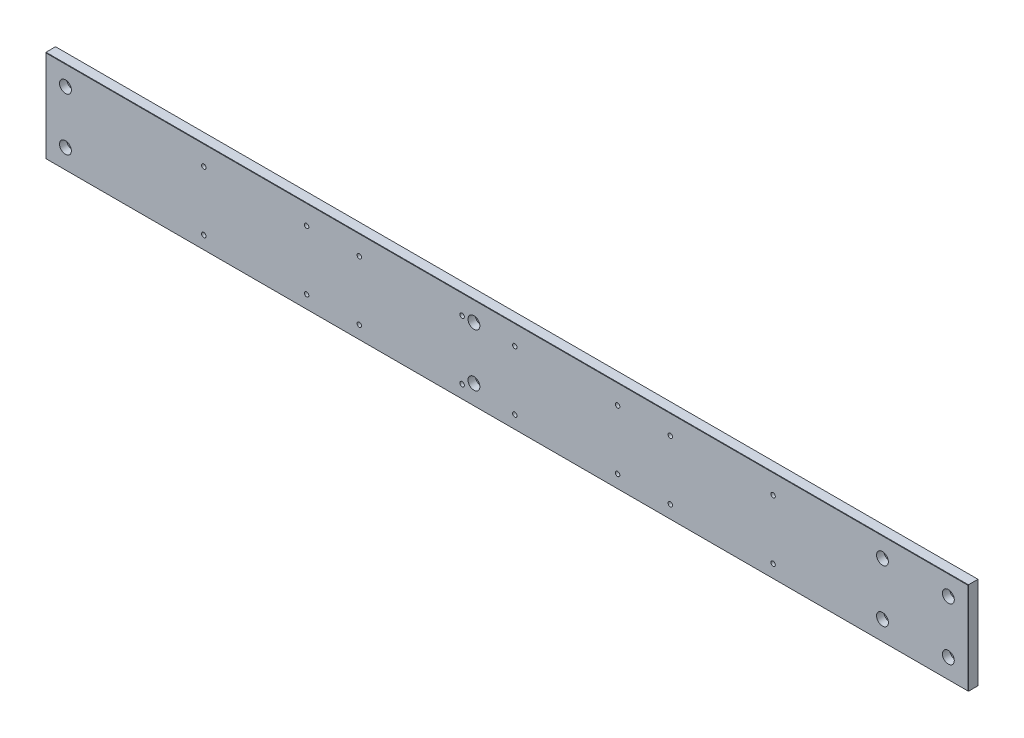
SolidWorks part; units mm, degrees
material "普通碳钢"
ref_plane "前视基准面" through (0, 0, 0) normal (0, 0, 1) x (1, 0, 0)
ref_plane "上视基准面" through (0, 0, 0) normal (0, 1, 0) x (1, 0, 0)
ref_plane "右视基准面" through (0, 0, 0) normal (1, 0, 0) x (0, 0, -1)
sketch "草图1" plane through (0, 0, 0) normal (0, 0, 1) x (1, 0, 0)
  line L1 (-700, 70) -> (700, 70)
  line L2 (-700, 70) -> (-700, -70)
  line L3 (-700, -70) -> (700, -70)
  line L4 (700, 70) -> (700, -70)
  line L5 (-700, 70) -> (700, -70) construction
  line L6 (-700, -70) -> (700, 70) construction
  point P0 (0, 0)
  dimension "D1" = 1400
  dimension "D2" = 140
extrude "凸台-拉伸1" add sketch "草图1" along normal mid plane 15
hole_wizard "打孔尺寸(%根据)内六角圆柱头螺钉的类型1" positions "3D草图1" profile "草图2" counterbore size "M10" standard "GB" end condition through all
sketch3d "3D草图1"
  line L0 (700, 70, 7.5) -> (-700, 70, 7.5) construction
  line L1 (-700, 70, 7.5) -> (-700, -70, 7.5) construction
  point P0 (-670, 40, 7.5)
  dimension "D1" = 30
  dimension "D2" = 30
sketch "草图2" plane through (-670, 40, 7.5) normal (1, 0, 0) x (0, -1, 0)
  line L0 (0, 0) -> (0, 15)
  line L1 (0, 15) -> (5.5, 15)
  line L3 (5.5, 15) -> (5.5, 11)
  line L4 (5.5, 11) -> (9, 11)
  line L5 (9, 11) -> (9, 0)
  line L7 (9, 0) -> (0, 0)
  line L11 (0, -6.35) -> (0, 107.95) construction
  dimension "通孔孔直径" = 11
  dimension "通孔孔深度" = 15
  dimension "柱形沉头孔直径" = 18
  dimension "柱形沉头孔深度" = 11
pattern_linear "阵列(线性)1" count 3 spacing 620 along (1, 0, 0) count 2 spacing 80 along (0, -1, 0) of "打孔尺寸(%根据)内六角圆柱头螺钉的类型1"
hole_wizard "打孔尺寸(%根据)内六角圆柱头螺钉的类型2" positions "3D草图2" profile "草图3" counterbore size "M10" standard "GB" end condition through all
sketch3d "3D草图2"
  line L0 (700, -70, 7.5) -> (700, 70, 7.5) construction
  line L1 (700, 70, 7.5) -> (-700, 70, 7.5) construction
  line L2 (-700, -70, 7.5) -> (700, -70, 7.5) construction
  point P0 (670, 40, 7.5)
  point P2 (670, -40, 7.5)
  dimension "D1" = 30
  dimension "D2" = 30
  dimension "D3" = 30
  dimension "D4" = 30
sketch "草图3" plane through (670, 40, 7.5) normal (1, 0, 0) x (0, -1, 0)
  line L0 (0, 0) -> (0, 15)
  line L1 (0, 15) -> (5.5, 15)
  line L3 (5.5, 15) -> (5.5, 11)
  line L4 (5.5, 11) -> (9, 11)
  line L5 (9, 11) -> (9, 0)
  line L7 (9, 0) -> (0, 0)
  line L11 (0, -6.35) -> (0, 107.95) construction
  dimension "通孔孔直径" = 11
  dimension "通孔孔深度" = 15
  dimension "柱形沉头孔直径" = 18
  dimension "柱形沉头孔深度" = 11
chamfer "倒角1" distance 0.5 angle 45 4 edges at (700, 0, 7.5) (0, -70, 7.5) (-700, 0, 7.5) (0, 70, 7.5)
hole_wizard "M8 螺纹孔1" positions "草图10" profile "草图9" tap size "M8" standard "GB" end condition through all
sketch "草图10" plane through (0, 0, 7.5) normal (0, 0, 1) x (1, 0, 0)
  line L2 (700, -70) -> (-700, -70) construction
  line L3 (-700, -70) -> (-700, 70) construction
  point P0 (-460, 40)
  point P2 (-460, -50)
  point P4 (-304, -50)
  point P6 (-304, 40)
  point P17 (-224, 40)
  point P18 (-224, -50)
  point P19 (-68, -50)
  point P20 (-68, 40)
  point P21 (12, 40)
  point P22 (12, -50)
  point P23 (168, -50)
  point P24 (168, 40)
  point P25 (248, 40)
  point P26 (248, -50)
  point P27 (404, -50)
  point P28 (404, 40)
  dimension "D1" = 20
  dimension "D2" = 240
  dimension "D3" = 156
  dimension "D4" = 90
  dimension "D5" = 4
sketch "草图9" plane through (-460, 40, 7.5) normal (1, 0, 0) x (0, -1, 0)
  line L0 (0, 0) -> (0, 15)
  line L1 (0, 15) -> (3.4, 15)
  line L2 (3.4, 15) -> (3.4, 0)
  line L5 (3.4, 0) -> (0, 0)
  line L11 (0, -6.35) -> (0, 107.95) construction
  dimension "通孔螺纹孔钻头直径" = 6.8
  dimension "通孔螺纹孔钻头深度" = 15
cosmetic thread "孔螺蚊线1" parameters "D2"=8
cosmetic thread "孔螺蚊线2" parameters "D2"=8
cosmetic thread "孔螺蚊线3" parameters "D2"=8
cosmetic thread "孔螺蚊线4" parameters "D2"=8
cosmetic thread "孔螺蚊线5" parameters "D2"=8
cosmetic thread "孔螺蚊线6" parameters "D2"=8
cosmetic thread "孔螺蚊线7" parameters "D2"=8
cosmetic thread "孔螺蚊线8" parameters "D2"=8
cosmetic thread "孔螺蚊线9" parameters "D2"=8
cosmetic thread "孔螺蚊线10" parameters "D2"=8
cosmetic thread "孔螺蚊线11" parameters "D2"=8
cosmetic thread "孔螺蚊线12" parameters "D2"=8
cosmetic thread "孔螺蚊线13" parameters "D2"=8
cosmetic thread "孔螺蚊线14" parameters "D2"=8
cosmetic thread "孔螺蚊线15" parameters "D2"=8
cosmetic thread "孔螺蚊线16" parameters "D2"=8
